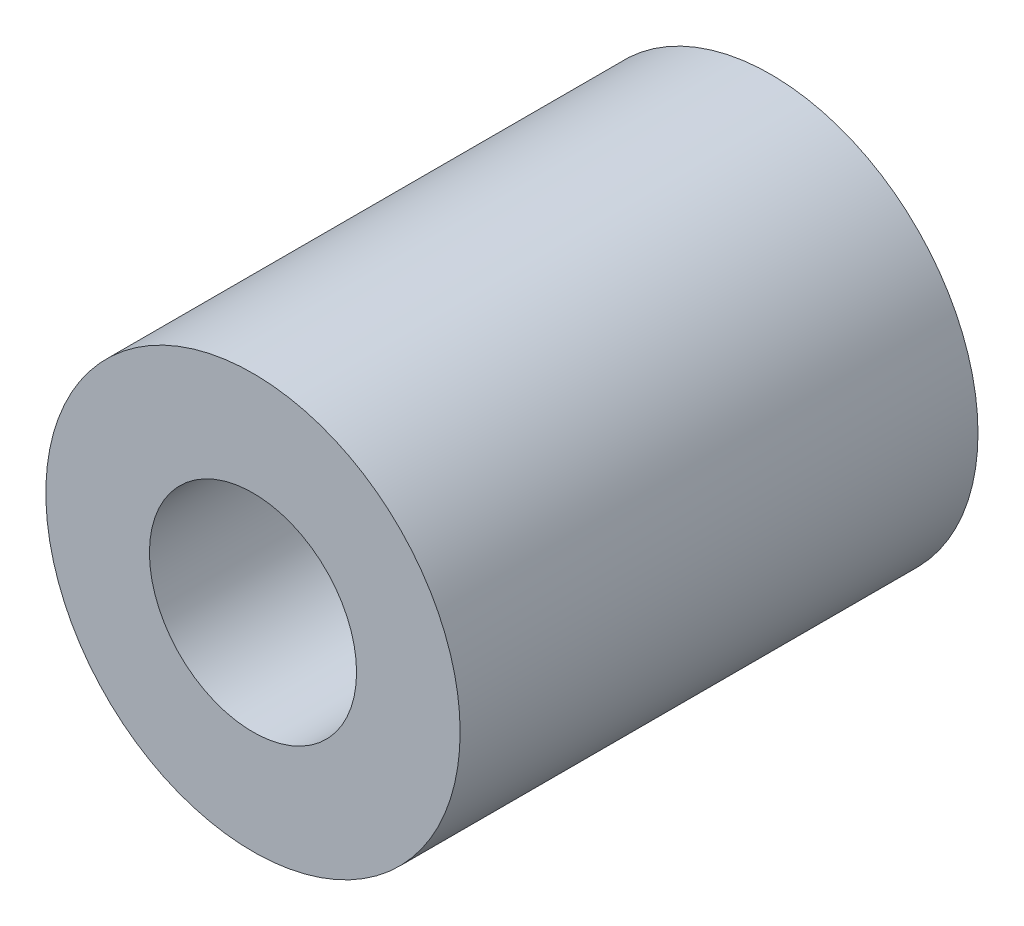
from build123d import *

# Parameters (mm, degrees)
SKETCH_1_R                = 6
EXTRUDE_1_DEPTH           = 15
HOLE_WIZARD_1_D           = 3.3
HOLE_WIZARD_1_CBORE_D     = 6
HOLE_WIZARD_1_CBORE_DEPTH = 10


with BuildPart() as part:
    # 草图1 → 凸台-拉伸1 (new body)
    with BuildSketch(Plane.XY):
        Circle(SKETCH_1_R)
    extrude(amount=EXTRUDE_1_DEPTH)

    # 打孔尺寸(%根据)内六角圆柱头螺钉的类型1 (through all)
    with Locations(Plane.XY.offset(15)):
        with Locations((0, 0)):
            CounterBoreHole(HOLE_WIZARD_1_D / 2, HOLE_WIZARD_1_CBORE_D / 2, HOLE_WIZARD_1_CBORE_DEPTH)


solid = part.part
